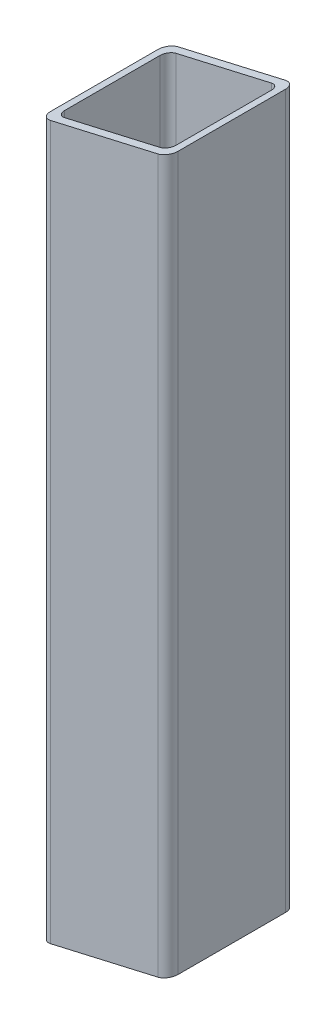
SolidWorks part; units mm, degrees
material "Angle steel 100×100×6/Q235"
ref_plane "Front Plane" through (0, 0, 0) normal (0, 0, 1) x (1, 0, 0)
ref_plane "Top Plane" through (0, 0, 0) normal (0, 1, 0) x (1, 0, 0)
ref_plane "Right Plane" through (0, 0, 0) normal (1, 0, 0) x (0, 0, -1)
sketch "Sketch2" plane through (0, 0, 0) normal (0, 1, 0) x (1, 0, 0)
  line L0 (12.6, 4.775) -> (87.4, 4.775)
  line L1 (6.3, 11.075) -> (6.3, 85.875)
  line L2 (87.4, 92.175) -> (12.6, 92.175)
  line L3 (93.7, 85.875) -> (93.7, 11.075)
  line L4 (7.875, -1.525) -> (92.125, -1.525)
  line L5 (0, 6.35) -> (0, 90.6)
  line L6 (92.125, 98.475) -> (7.875, 98.475)
  line L7 (100, 90.6) -> (100, 6.35)
  arc A0 (100, 90.6) -> (92.125, 98.475) centre (92.125, 90.6) ccw
  arc A1 (92.125, -1.525) -> (100, 6.35) centre (92.125, 6.35) ccw
  arc A2 (0, 6.35) -> (7.875, -1.525) centre (7.875, 6.35) ccw
  arc A3 (7.875, 98.475) -> (0, 90.6) centre (7.875, 90.6) ccw
  arc A4 (12.6, 92.175) -> (6.3, 85.875) centre (12.6, 85.875) ccw
  arc A5 (93.7, 85.875) -> (87.4, 92.175) centre (87.4, 85.875) ccw
  arc A6 (87.4, 4.775) -> (93.7, 11.075) centre (87.4, 11.075) ccw
  arc A7 (6.3, 11.075) -> (12.6, 4.775) centre (12.6, 11.075) ccw
extrude "Boss-Extrude1" add sketch "Sketch2" along normal mid plane 582
sketch "Sketch4" plane through (0, 0, 1.525) normal (0, 0, 1) x (1, 0, 0)
  line L0 (100, 291) -> (0, 268)
  line L1 (0, 291) -> (0, -291) construction
  line L2 (0, 268) -> (0, 291)
  line L3 (0, 291) -> (100, 291)
  line L4 (0, -291) -> (100, -268)
  line L5 (100, 291) -> (100, -291) construction
  line L6 (100, -268) -> (100, -291)
  line L7 (100, -291) -> (0, -291)
  dimension "D1" = 23
  dimension "D2" = 23
  dimension "D3" = 559
  dimension "D4" = 559
extrude "Cut-Extrude1" cut sketch "Sketch4" against normal up to next
